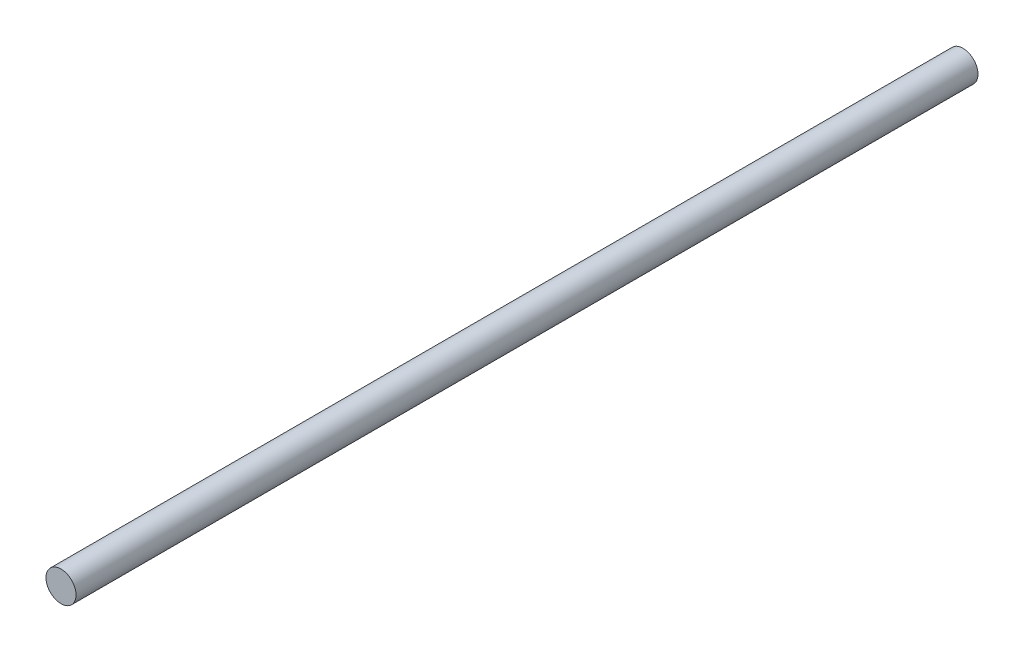
from build123d import *

# Parameters (mm, degrees)
SKETCH_1_R      = 10
EXTRUDE_1_DEPTH = 300


with BuildPart() as part:
    # 草图1 → 凸台-拉伸1 (new, symmetric)
    with BuildSketch(Plane.XY):
        Circle(SKETCH_1_R)
    extrude(amount=EXTRUDE_1_DEPTH, both=True)


solid = part.part
